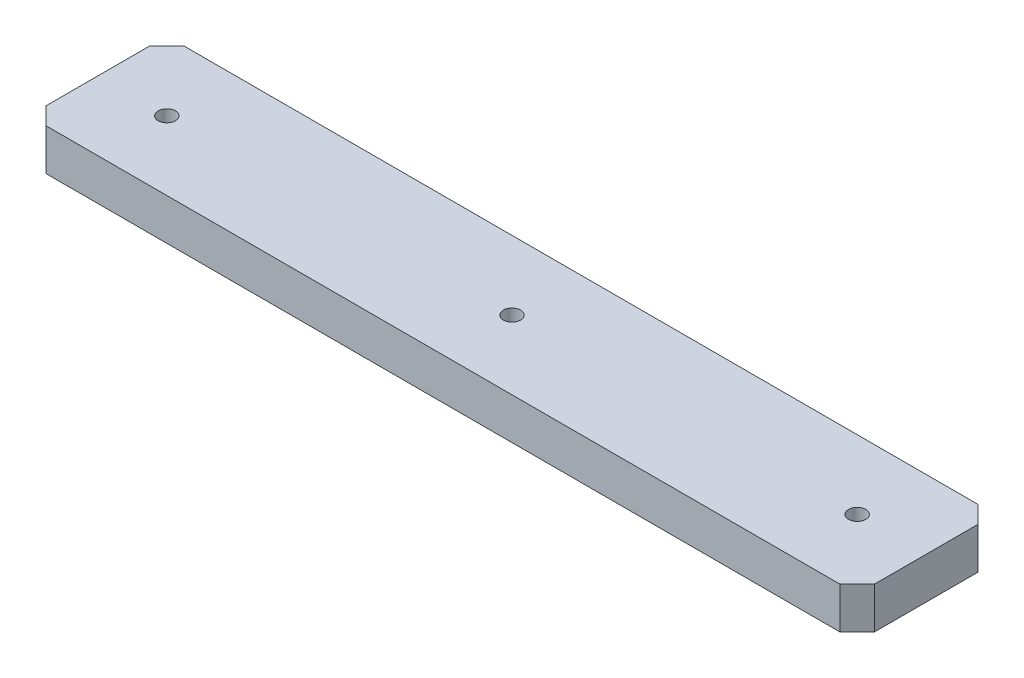
SolidWorks part; units mm, degrees
material "45#"
ref_plane "Front Plane" through (0, 0, 0) normal (0, 0, 1) x (1, 0, 0)
ref_plane "Top Plane" through (0, 0, 0) normal (0, 1, 0) x (1, 0, 0)
ref_plane "Right Plane" through (0, 0, 0) normal (1, 0, 0) x (0, 0, -1)
sketch "Sketch1" plane through (0, 0, 0) normal (0, 1, 0) x (1, 0, 0)
  line L0 (120, 20) -> (-120, -20) construction
  line L1 (-120, 20) -> (120, 20)
  line L2 (-120, 20) -> (-120, -20)
  line L3 (-120, -20) -> (120, -20)
  line L4 (120, 20) -> (120, -20)
  dimension "D1" = 240
  dimension "D2" = 40
extrude "Extrude1" add sketch "Sketch1" along normal mid plane 12
hole_wizard "M6 Tapped Hole1" positions "Sketch3" profile "Sketch2" tap size "M6" standard "ISO"
sketch "Sketch3" plane through (0, 6, 0) normal (0, 1, 0) x (-1, 0, 0)
  line L0 (-100, 0) -> (0, 0) construction
  line L1 (0, 0) -> (100, 0) construction
  line L3 (-120, 20) -> (-120, -20) construction
  point P0 (100, 0)
  point P1 (0, 0)
  point P3 (-100, 0)
  dimension "D1" = 20
sketch "Sketch2" plane through (-100, 6, 0) normal (1, 0, 0) x (0, 0, 1)
  line L0 (0, 0) -> (0, 16.5022)
  line L1 (0, 16.5022) -> (2.5, 15)
  line L2 (2.5, 15) -> (2.5, 0)
  line L5 (2.5, 0) -> (0, 0)
  line L10 (0, 16.5022) -> (-2.5, 15) construction
  line L11 (0, -6.35) -> (0, 107.95) construction
  dimension "螺孔鑽直徑" = 5
  dimension "螺孔鑽深度" = 15
  dimension "導頭角度" = 118
cosmetic thread "Cosmetic Thread1" parameters "D1"=12, "D2"=6
cosmetic thread "Cosmetic Thread2" parameters "D1"=12, "D2"=6
cosmetic thread "Cosmetic Thread3" parameters "D1"=12, "D2"=6
chamfer "Chamfer1" distance 5 angle 45 4 edges at (120, 0, 20) (-120, 0, 20) (-120, 0, -20) (120, 0, -20)
